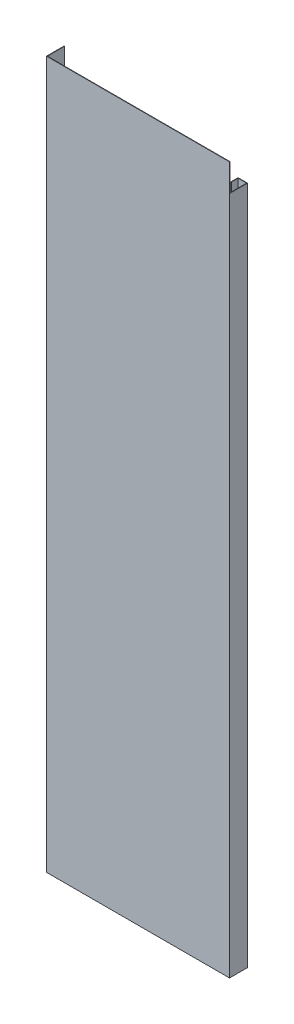
from build123d import *

# Parameters (mm, degrees)
EXTRUDE_THIN1_DEPTH = 1649
SKETCH4_W           = 22
SKETCH4_H           = 64
CUT_EXTRUDE1_DEPTH  = 41


with BuildPart() as part:
    # Sketch3 → Extrude-Thin1 (new body)
    with BuildSketch(Plane(origin=(0, 0, 0), x_dir=(1, 0, 0), z_dir=(0, 1, 0))):
        Polygon((0, 40), (0, 0), (425, 0), (425, 40), (405, 40), (405, 25), (404, 25), (404, 41), (426, 41), (426, -1), (-1, -1), (-1, 40), align=None)
    extrude(amount=EXTRUDE_THIN1_DEPTH)

    # Sketch4 → Cut-Extrude1 (cut)
    with BuildSketch(Plane(origin=(0, 0, -41), x_dir=(-1, 0, 0), z_dir=(0, 0, -1))):
        with Locations((-415, 1617)):
            Rectangle(SKETCH4_W, SKETCH4_H)
    extrude(amount=-CUT_EXTRUDE1_DEPTH, mode=Mode.SUBTRACT)


solid = part.part
